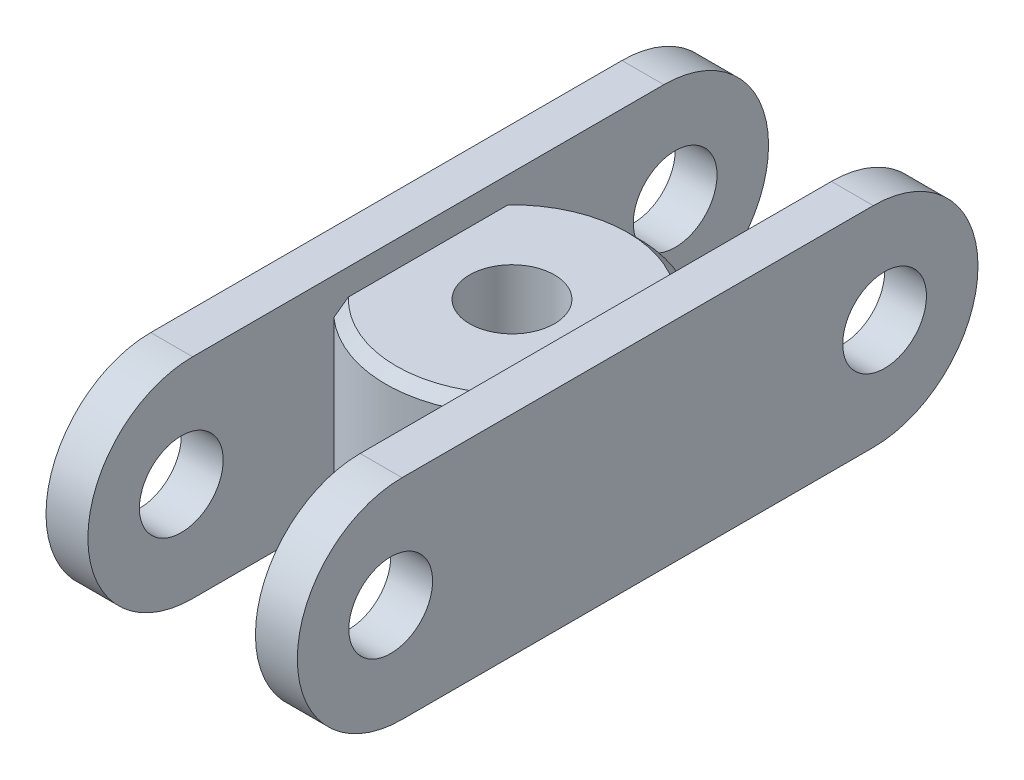
from build123d import *

# Parameters (mm, degrees)
SKETCH1_R          = 12.05
SKETCH1_R_2        = 4.05
BOSS_EXTRU_1_DEPTH = 15
CHAMFER1_SIZE      = 1
CUT_EXTRUDE1_REACH = 24.703
SKETCH5_W          = 7
SKETCH5_H          = 40.880501257
SKETCH6_R          = 4
BOSS_EXTRU_4_DEPTH = 4


with BuildPart() as part:
    # Sketch1 → Boss.-Extru.1 (new body)
    with BuildSketch(Plane(origin=(0, 0, 0), x_dir=(1, 0, 0), z_dir=(0, 1, 0))):
        with Locations(Location((0, 0, 0), (0, 0, 270))):
            Circle(SKETCH1_R)
        with Locations(Location((0, 0, 0), (0, 0, 270))):
            Circle(SKETCH1_R_2, mode=Mode.SUBTRACT)
    extrude(amount=BOSS_EXTRU_1_DEPTH)

    # Chamfer1
    chamfer1_edges = [part.edges().sort_by_distance(p)[0] for p in [
        (0, 15, -12.05),
    ]]
    chamfer(chamfer1_edges, length=CHAMFER1_SIZE)

    # Sketch5 → Cut-Extrude1 (cut, up to next)
    with BuildSketch(Plane(origin=(0, 15, 0), x_dir=(1, 0, 0), z_dir=(0, 1, 0)), mode=Mode.PRIVATE) as cut_extrude1_sk1:
        with Locations((11.5, -1.662295536)):
            Rectangle(SKETCH5_W, SKETCH5_H)
    cut_extrude1_tool1 = extrude(cut_extrude1_sk1.sketch, amount=-CUT_EXTRUDE1_REACH, mode=Mode.PRIVATE) & part.part
    # Sketch5 → Cut-Extrude1 (cut, up to next)
    with BuildSketch(Plane(origin=(0, 15, 0), x_dir=(1, 0, 0), z_dir=(0, 1, 0)), mode=Mode.PRIVATE) as cut_extrude1_sk2:
        with Locations((-11.5, -1.662295536)):
            Rectangle(SKETCH5_W, SKETCH5_H)
    cut_extrude1_tool2 = extrude(cut_extrude1_sk2.sketch, amount=-CUT_EXTRUDE1_REACH, mode=Mode.PRIVATE) & part.part
    add(cut_extrude1_tool1.solids().sort_by_distance((11.5, 15, 1.662296))[0], mode=Mode.SUBTRACT)
    add(cut_extrude1_tool2.solids().sort_by_distance((-11.5, 15, 1.662296))[0], mode=Mode.SUBTRACT)

    # Sketch6 → Boss.-Extru.4 (add)
    with BuildSketch(Plane(origin=(8, 0, 0), x_dir=(0, 0, -1), z_dir=(1, 0, 0))):
        with BuildLine():
            Line((22.5, -2.5), (-22.5, -2.5))
            ThreePointArc((-22.5, -2.5), (-32.5, 7.5), (-22.5, 17.5))
            Line((-22.5, 17.5), (22.5, 17.5))
            ThreePointArc((22.5, 17.5), (32.5, 7.5), (22.5, -2.5))
        make_face()
        with Locations((23.579898115, 7.5)):
            Circle(SKETCH6_R, mode=Mode.SUBTRACT)
        with Locations(Location((-23.579898115, 7.5, 0), (0, 0, 180))):
            Circle(SKETCH6_R, mode=Mode.SUBTRACT)
    boss_extru_4 = extrude(amount=BOSS_EXTRU_4_DEPTH)

    # Mirror1: Boss.-Extru.4 across plane
    add(boss_extru_4.mirror(Plane(origin=(0, 0, 0), x_dir=(0, 0, 1), z_dir=(1, 0, 0))))


solid = part.part
